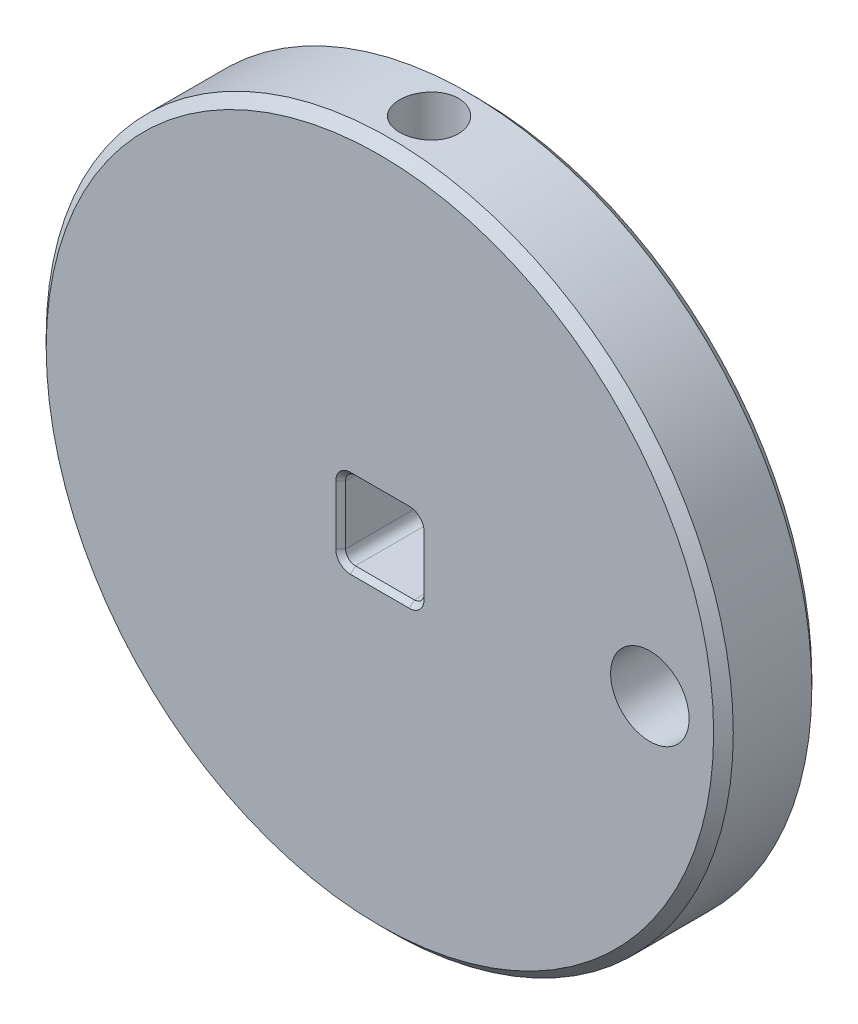
from build123d import *

# Parameters (mm, degrees)
SKETCH1_R             = 35
BOSS_EXTRUDE1_DEPTH   = 10
CHAMFER1_SIZE         = 1
SKETCH2_R             = 1
CUT_EXTRUDE1_DEPTH    = 30
SKETCH3_R             = 4
CUT_EXTRUDE2_DEPTH    = 29
SKETCH4_W             = 8
SKETCH4_H             = 8
CUT_EXTRUDE3_DEPTH    = 51.497524692
FILLET1_R             = 1
SKETCH5_R             = 0.5
CUT_EXTRUDE4_DEPTH    = 54.347914673
SKETCH7_R             = 3
CUT_EXTRUDE5_DEPTH    = 62.040969986
M3_TAPPED_HOLE1_D     = 2.5
M3_TAPPED_HOLE1_DEPTH = 12
M3_TAPPED_HOLE1_TIP   = 0.751075774
CHAMFER2_SIZE         = 0.5


with BuildPart() as part:
    # Sketch1 → Boss-Extrude1 (new body)
    with BuildSketch(Plane.XY):
        Circle(SKETCH1_R)
    extrude(amount=BOSS_EXTRUDE1_DEPTH)

    # Chamfer1
    chamfer1_edges = [part.edges().sort_by_distance(p)[0] for p in [
        (-35, 0, 0),
        (-35, 0, 10),
    ]]
    chamfer(chamfer1_edges, length=CHAMFER1_SIZE)

    # Sketch2 → Cut-Extrude1 (cut)
    with BuildSketch(Plane.XY.offset(10)):
        Circle(SKETCH2_R)
    extrude(amount=-CUT_EXTRUDE1_DEPTH, mode=Mode.SUBTRACT)

    # Sketch3 → Cut-Extrude2 (cut)
    with BuildSketch(Plane.XY.offset(10)):
        with Locations((27.5, 0)):
            Circle(SKETCH3_R)
    extrude(amount=-CUT_EXTRUDE2_DEPTH, mode=Mode.SUBTRACT)

    # Sketch4 → Cut-Extrude3 (cut, through all)
    with BuildSketch(Plane.XY.offset(10)):
        Rectangle(SKETCH4_W, SKETCH4_H)
    extrude(amount=-CUT_EXTRUDE3_DEPTH, mode=Mode.SUBTRACT)

    # Fillet1
    fillet1_edges = [part.edges().sort_by_distance(p)[0] for p in [
        (4, 4, 5),
        (4, -4, 5),
        (-4, -4, 5),
        (-4, 4, 5),
    ]]
    fillet(fillet1_edges, radius=FILLET1_R)

    # Sketch5 → Cut-Extrude4 (cut, through all)
    with BuildSketch(Plane.XZ.offset(-4)):
        with Locations(Location((0, 5, 0), (0, 0, 270))):
            Circle(SKETCH5_R)
    extrude(amount=-CUT_EXTRUDE4_DEPTH, mode=Mode.SUBTRACT)

    # Sketch7 → Cut-Extrude5 (cut, through all)
    with BuildSketch(Plane(origin=(0, 14, 0), x_dir=(1, 0, 0), z_dir=(0, 1, 0))):
        with Locations(Location((0, -5, 0), (0, 0, 90))):
            Circle(SKETCH7_R)
    extrude(amount=CUT_EXTRUDE5_DEPTH, mode=Mode.SUBTRACT)

    # M3 Tapped Hole1
    with Locations(Plane(origin=(0, 14, 5), x_dir=(0, 0, 1), z_dir=(0, 1, 0))):
        with Locations((0, 0)):
            Hole(M3_TAPPED_HOLE1_D / 2, depth=M3_TAPPED_HOLE1_DEPTH)
            with Locations((0, 0, -(M3_TAPPED_HOLE1_DEPTH + M3_TAPPED_HOLE1_TIP / 2))):  # 118° drill point
                Cone(0, M3_TAPPED_HOLE1_D / 2, M3_TAPPED_HOLE1_TIP, mode=Mode.SUBTRACT)

    # Chamfer2
    chamfer2_edges = [part.edges().sort_by_distance(p)[0] for p in [
        (0, -4, 10),
        (0, -4, 0),
        (-4, 0, 10),
        (-4, 0, 0),
        (4, 0, 10),
        (4, 0, 0),
        (0, 4, 10),
        (0, 4, 0),
        (-3.707106781, -3.707106781, 10),
        (-3.707106781, -3.707106781, 0),
        (3.707106781, -3.707106781, 10),
        (3.707106781, -3.707106781, 0),
        (3.707106781, 3.707106781, 10),
        (3.707106781, 3.707106781, 0),
        (-3.707106781, 3.707106781, 10),
        (-3.707106781, 3.707106781, 0),
    ]]
    chamfer(chamfer2_edges, length=CHAMFER2_SIZE)


solid = part.part
